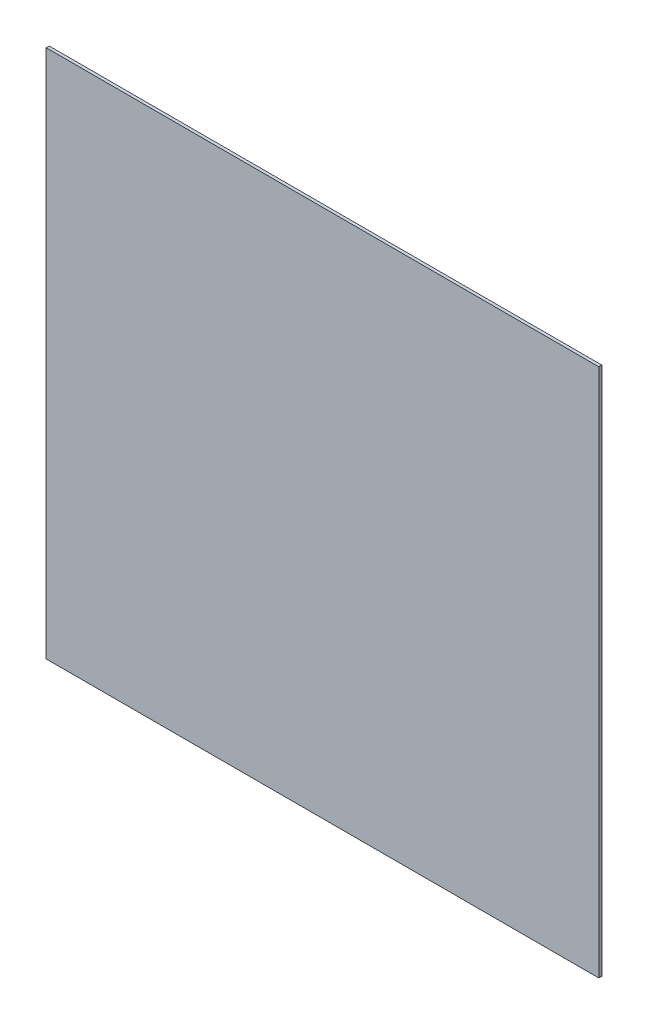
SolidWorks part; units mm, degrees
material "PMMA(有机玻璃)"
ref_plane "前视" through (0, 0, 0) normal (0, 0, 1) x (1, 0, 0)
ref_plane "上视" through (0, 0, 0) normal (0, 1, 0) x (1, 0, 0)
ref_plane "右视" through (0, 0, 0) normal (1, 0, 0) x (0, 0, -1)
sketch "草图1" plane through (0, 0, 0) normal (0, 0, 1) x (1, 0, 0)
  line L1 (-463, 443.5) -> (463, 443.5)
  line L2 (-463, 443.5) -> (-463, -443.5)
  line L3 (-463, -443.5) -> (463, -443.5)
  line L4 (463, 443.5) -> (463, -443.5)
  line L5 (-463, 443.5) -> (463, -443.5) construction
  line L6 (-463, -443.5) -> (463, 443.5) construction
  point P0 (0, 0)
  dimension "D1" = 887
  dimension "D2" = 926
extrude "凸台-拉伸1" add sketch "草图1" along normal blind 5
